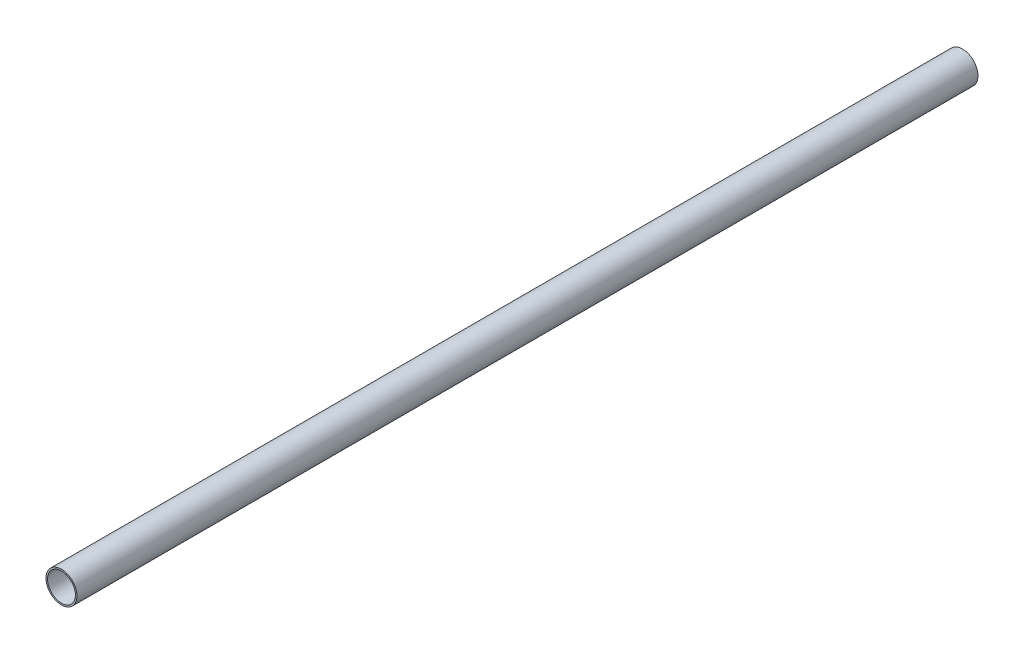
from build123d import *

# Parameters (mm, degrees)
SKETCH1_R           = 14.45
SKETCH1_R_2         = 13
BOSS_EXTRUDE1_DEPTH = 840


with BuildPart() as part:
    # Sketch1 → Boss-Extrude1 (new body)
    with BuildSketch(Plane.XY):
        Circle(SKETCH1_R)
        Circle(SKETCH1_R_2, mode=Mode.SUBTRACT)
    extrude(amount=BOSS_EXTRUDE1_DEPTH)


solid = part.part
